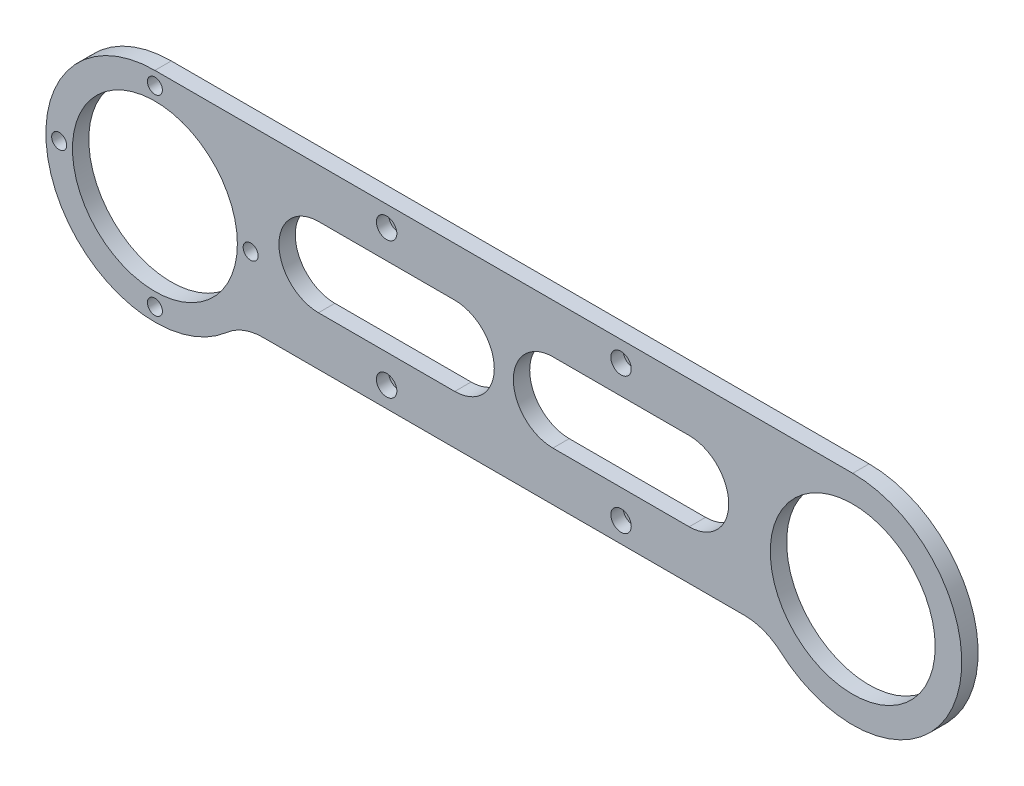
SolidWorks part; units mm, degrees
material "6061-T6 (SS)"
ref_plane "前视基准面" through (0, 0, 0) normal (0, 0, 1) x (1, 0, 0)
ref_plane "上视基准面" through (0, 0, 0) normal (0, 1, 0) x (1, 0, 0)
ref_plane "右视基准面" through (0, 0, 0) normal (1, 0, 0) x (0, 0, -1)
other "Configuration Table"
sketch "草图1" plane through (0, 0, 0) normal (0, 0, 1) x (1, 0, 0)
  line L1 (-256, 85.6685) -> (256, 85.6685)
  line L3 (-176.6275, -44.3315) -> (176.6275, -44.3315)
  line L9 (36, 20.6685) -> (136, 20.6685) construction
  line L10 (36, 49.6685) -> (136, 49.6685)
  line L13 (-136, 20.6685) -> (-36, 20.6685) construction
  line L14 (-136, 49.6685) -> (-36, 49.6685)
  line L15 (-136, -8.3315) -> (-36, -8.3315)
  line L16 (36, -8.3315) -> (136, -8.3315)
  arc A0 (-256, 85.6685) -> (-203.085, -54.3315) centre (-256, 5.6685) ccw
  arc A1 (203.085, -54.3315) -> (256, 85.6685) centre (256, 5.6685) ccw
  arc A2 (-203.085, -54.3315) -> (-176.6275, -44.3315) centre (-176.6275, -84.3315) cw
  arc A3 (203.085, -54.3315) -> (176.6275, -44.3315) centre (176.6275, -84.3315) ccw
  circle A4 centre (-256, 5.6685) radius 60.5
  arc A6 (-136, 49.6685) -> (-136, -8.3315) centre (-136, 20.6685) ccw
  arc A7 (-36, -8.3315) -> (-36, 49.6685) centre (-36, 20.6685) ccw
  arc A8 (36, 49.6685) -> (36, -8.3315) centre (36, 20.6685) ccw
  arc A9 (136, -8.3315) -> (136, 49.6685) centre (136, 20.6685) ccw
  point P4 (0, 0)
  point P13 (0, -50)
  point P17 (-86, 20.6685)
  point P22 (86, 20.6685)
  dimension "D2" = 160
  dimension "D3" = 160
  dimension "D5" = 40
  dimension "D6" = 40
  dimension "D7" = 121
  dimension "D1" = 512
  dimension "D4" = 58
  dimension "D10" = 100
  dimension "D11" = 100
  dimension "D13" = 58
extrude "凸台-拉伸2" add sketch "草图1" along normal blind 12
sketch "草图3" plane through (0, 0, 0) normal (0, 0, 1) x (1, 0, 0)
  circle A1 centre (256, 5.6685) radius 60.5
  dimension "D2" = 121
extrude "切除-拉伸2" cut sketch "草图3" along normal through all from offset 8
sketch "草图5" plane through (0, 0, 0) normal (0, 0, 1) x (1, 0, 0)
  circle A2 centre (256, 5.6685) radius 18
  dimension "D1" = 36
extrude "切除-拉伸3" cut sketch "草图5" along normal through all
sketch "草图6" plane through (0, 0, 0) normal (0, 0, 1) x (1, 0, 0)
  line L0 (-86, 49.6685) -> (-86, 70.6685)
  line L1 (-36, 49.6685) -> (-136, 49.6685) construction
  line L5 (-86, -9.7199) -> (-86, -29.3315)
  line L11 (86, 49.6685) -> (86, 70.6685)
  line L12 (136, 49.6685) -> (36, 49.6685) construction
  line L13 (86, -29.3315) -> (86, -9.7199)
  point P17 (-86, 20.6685)
  point P26 (86, 20.6685)
  dimension "D1" = 100
  dimension "D2" = 100
hole_wizard "M8 六角圆柱头螺钉的柱形沉头孔1" positions "草图7" profile "草图8" counterbore size "M8" standard "GB" end condition through all
sketch "草图7" plane through (0, 0, 12) normal (0, 0, 1) x (1, 0, 0)
  point P0 (-86, 70.6685)
  point P3 (-86, -29.3315)
  point P6 (86, 70.6685)
  point P9 (86, -29.3315)
sketch "草图8" plane through (-86, 70.6685, 12) normal (1, 0, 0) x (0, -1, 0)
  line L0 (0, 0) -> (0, 12)
  line L1 (0, 12) -> (4.5, 12)
  line L3 (4.5, 12) -> (4.5, 9)
  line L4 (4.5, 9) -> (7.5, 9)
  line L5 (7.5, 9) -> (7.5, 0)
  line L7 (7.5, 0) -> (0, 0)
  line L11 (0, -6.35) -> (0, 107.95) construction
  dimension "通孔孔直径" = 9
  dimension "通孔孔深度" = 12
  dimension "柱形沉头孔直径" = 15
  dimension "柱形沉头孔深度" = 9
sketch "草图9" plane through (0, 0, 0) normal (0, 0, -1) x (-1, 0, 0)
  circle A17 centre (256, 5.6685) radius 70.25 construction
  circle A18 centre (256, 75.9185) radius 5.5
  circle A19 centre (326.25, 5.6685) radius 5.5
  circle A20 centre (256, -64.5815) radius 5.5
  circle A21 centre (185.75, 5.6685) radius 5.5
  point P14 (256, 5.6685)
  point P28 (256, 5.6685)
  dimension "D1" = 11
  dimension "D3" = 140.5
  dimension "D2" = 4
extrude "切除-拉伸4" cut sketch "草图9" against normal through all
sketch "草图10" plane through (0, 0, 8) normal (0, 0, 1) x (1, 0, 0)
  circle A0 centre (256, 5.6685) radius 60.5
extrude "切除-拉伸5" cut sketch "草图10" against normal through all
